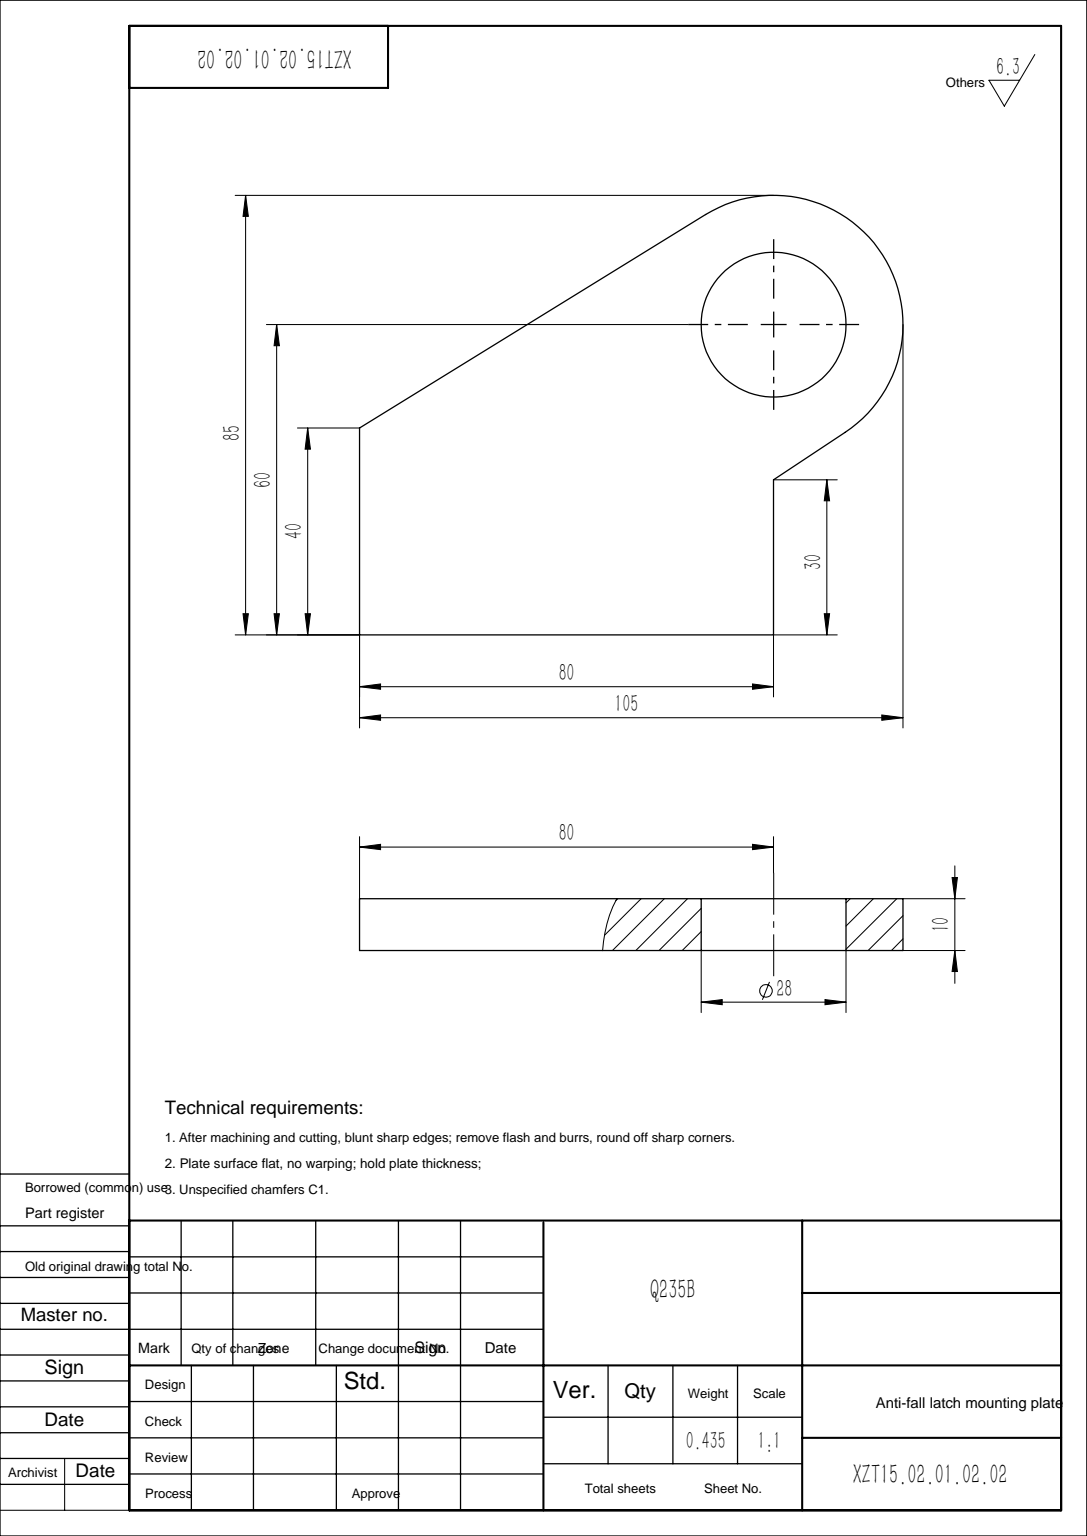
SolidWorks part; units mm, degrees
material "Q235B"
ref_plane "Front Plane" through (0, 0, 0) normal (0, 0, 1) x (1, 0, 0)
ref_plane "Top Plane" through (0, 0, 0) normal (0, 1, 0) x (1, 0, 0)
ref_plane "Right Plane" through (0, 0, 0) normal (1, 0, 0) x (0, 0, -1)
sketch "Sketch1" plane through (0, 0, 0) normal (0, 0, 1) x (1, 0, 0)
  line L0 (0, 0) -> (0, 40)
  line L1 (0, 40) -> (66.869, 81.2739)
  line L2 (80, 30) -> (80, 0)
  line L3 (80, 0) -> (0, 0)
  line L4 (80, 30) -> (93.8193, 39.1667)
  circle A1 centre (80, 60) radius 14
  arc A2 (66.869, 81.2739) -> (93.8193, 39.1667) centre (80, 60) cw
  dimension "D1" = 80
  dimension "D3" = 85
  dimension "D6" = 28
  dimension "D7" = 105
  dimension "D2" = 30
  dimension "D4" = 60
  dimension "D5" = 40
extrude "Boss-Extrude1" add sketch "Sketch1" along normal mid plane 10
